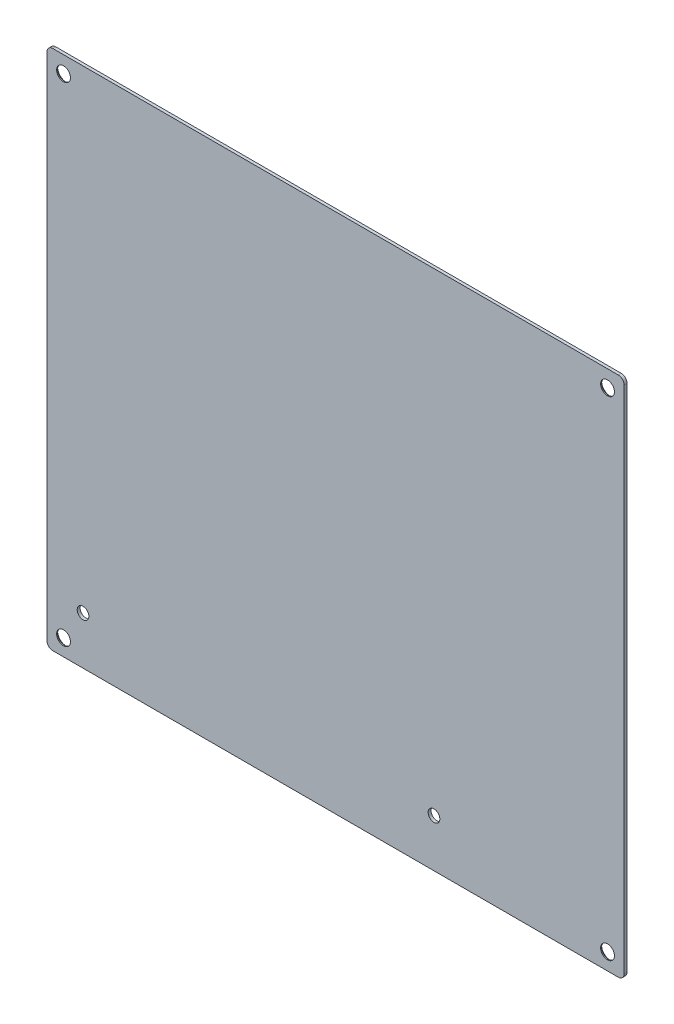
SolidWorks part; units mm, degrees
ref_plane "前视基准面" through (0, 0, 0) normal (0, 0, 1) x (1, 0, 0)
ref_plane "上视基准面" through (0, 0, 0) normal (0, 1, 0) x (1, 0, 0)
ref_plane "右视基准面" through (0, 0, 0) normal (1, 0, 0) x (0, 0, -1)
sketch "草图1" plane through (0, 0, 0) normal (0, 0, 1) x (1, 0, 0)
  line L0 (-89.5, 67) -> (-89.5, 334.5)
  line L1 (-89.5, 334.5) -> (-385.5, 334.5)
  line L2 (-385.5, 334.5) -> (-385.5, 67)
  line L3 (-385.5, 67) -> (-89.5, 67)
extrude "凸台-拉伸1" add sketch "草图1" against normal blind 1.5
fillet "圆角1" radius 3 4 edges at (-89.5, 67, -0.75) (-89.5, 334.5, -0.75) (-385.5, 67, -0.75) (-385.5, 334.5, -0.75)
sketch "草图6" plane through (0, 0, 0) normal (0, 0, 1) x (1, 0, 0)
  line L0 (-382.5, 67) -> (-92.5, 67) construction
  line L1 (-385.5, 331.5) -> (-385.5, 70) construction
  circle A0 centre (-367, 91.5) radius 3
  circle A1 centre (-187, 91.5) radius 3
  dimension "D1" = 6
  dimension "D2" = 24.5
  dimension "D3" = 18.5
  dimension "D4" = 6
  dimension "D5" = 180
extrude "切除-拉伸1" cut sketch "草图6" against normal blind 1.5
sketch "草图7" plane through (0, 0, -1.5) normal (0, 0, -1) x (-1, 0, 0)
  line L0 (89.5, 70) -> (89.5, 331.5) construction
  line L1 (92.5, 334.5) -> (382.5, 334.5) construction
  line L2 (385.5, 331.5) -> (385.5, 70) construction
  line L3 (382.5, 67) -> (92.5, 67) construction
  circle A0 centre (98, 326) radius 3.55
  circle A1 centre (377, 326) radius 3.55
  circle A2 centre (377, 75.5) radius 3.55
  circle A3 centre (98, 75.5) radius 3.55
  dimension "D1" = 7.1
  dimension "D2" = 8.5
  dimension "D3" = 8.5
  dimension "D4" = 7.1
  dimension "D5" = 8.5
  dimension "D6" = 8.5
  dimension "D7" = 7.1
  dimension "D8" = 8.5
  dimension "D9" = 8.5
  dimension "D10" = 7.1
  dimension "D11" = 8.5
  dimension "D12" = 8.5
extrude "切除-拉伸2" cut sketch "草图7" against normal blind 1.5
chamfer "倒角1" distance 1 angle 45 4 edges at (-101.55, 326, -1.5) (-101.55, 75.5, -1.5) (-380.55, 75.5, -1.5) (-380.55, 326, -1.5)
